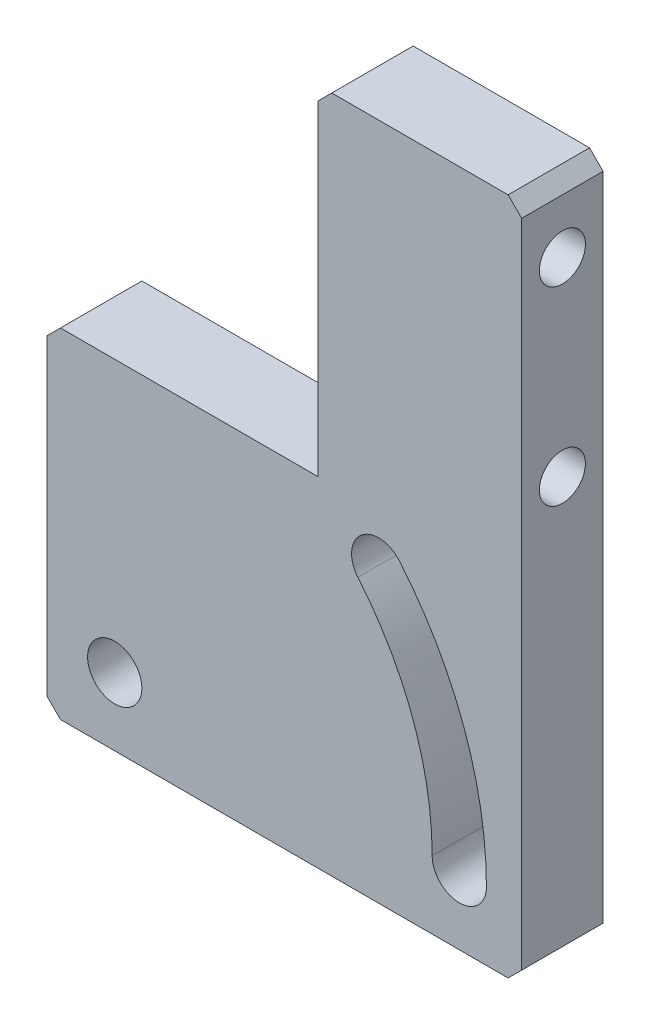
SolidWorks part; units mm, degrees
material "AL6061"
ref_plane "前视基准面" through (0, 0, 0) normal (0, 0, 1) x (1, 0, 0)
ref_plane "上视基准面" through (0, 0, 0) normal (0, 1, 0) x (1, 0, 0)
ref_plane "右视基准面" through (0, 0, 0) normal (1, 0, 0) x (0, 0, -1)
sketch "草图1" plane through (0, 0, 0) normal (0, 0, 1) x (1, 0, 0)
  line L1 (17.5, -25) -> (-17.5, -25)
  line L2 (17.5, -25) -> (17.5, 25)
  line L3 (17.5, 25) -> (-17.5, 25)
  line L4 (-17.5, -25) -> (-17.5, 25)
  line L5 (17.5, -25) -> (-17.5, 25) construction
  line L6 (17.5, 25) -> (-17.5, -25) construction
  point P0 (0, 0)
  dimension "D1" = 35
  dimension "D2" = 50
extrude "凸台-拉伸1" add sketch "草图1" along normal mid plane 6
sketch "草图2" plane through (0, 0, 3) normal (0, 0, 1) x (1, 0, 0)
  line L0 (17.5, -25) -> (17.5, 25) construction
  line L1 (-17.5, 25) -> (2.5, 25)
  line L2 (-17.5, 25) -> (-17.5, 0)
  line L3 (-17.5, 0) -> (2.5, 0)
  line L4 (2.5, 25) -> (2.5, 0)
  dimension "D1" = 15
  dimension "D2" = 25
extrude "切除-拉伸1" cut sketch "草图2" against normal through all
sketch "草图3" plane through (0, 0, 3) normal (0, 0, 1) x (1, 0, 0)
  line L0 (-17.5, 0) -> (-17.5, -25) construction
  line L1 (-17.5, -25) -> (17.5, -25) construction
  line L2 (-12.5, -20) -> (11.3682, -11.3127) construction
  line L3 (-12.5, -20) -> (0.9382, -20) construction
  line L4 (-12.5, -20) -> (12.9, -20) construction
  line L5 (-12.5, -20) -> (6.9575, -3.6732) construction
  circle A0 centre (-12.5, -20) radius 2
  arc A1 (6.9575, -3.6732) -> (12.9, -20) centre (-12.5, -20) cw construction
  arc A2 (14.9, -20) -> (8.4896, -2.3876) centre (-12.5, -20) ccw
  arc A3 (10.9, -20) -> (5.4254, -4.9588) centre (-12.5, -20) ccw
  arc A4 (10.9, -20) -> (14.9, -20) centre (12.9, -20) ccw
  arc A5 (8.4896, -2.3876) -> (5.4254, -4.9588) centre (6.9575, -3.6732) ccw
  point P4 (11.3682, -11.3127)
  dimension "D1" = 4
  dimension "D2" = 5
  dimension "D3" = 5
  dimension "D4" = 25.4
  dimension "D5" = 20
  dimension "D6" = 40
extrude "切除-拉伸2" cut sketch "草图3" against normal through all
sketch "草图4" plane through (2.5, 0, 0) normal (-1, 0, 0) x (0, 0, 1)
  line L0 (0, 25) -> (0, 20) construction
  line L1 (-3, 25) -> (3, 25) construction
  line L2 (0, 20) -> (0, 6) construction
  point P0 (0, 20)
  point P2 (0, 6)
  dimension "D1" = 5
  dimension "D2" = 14
hole_wizard "M3 间隙孔1" positions "草图4" profile "草图6" hole size "M3" standard "ISO" end condition through all
sketch "草图6" plane through (2.5, 20, 0) normal (0, 1, 0) x (0, 0, 1)
  line L0 (0, 0) -> (0, 15)
  line L1 (0, 15) -> (1.7, 15)
  line L2 (1.7, 15) -> (1.7, 0)
  line L5 (1.7, 0) -> (0, 0)
  line L11 (0, -6.35) -> (0, 107.95) construction
  dimension "通孔孔直径" = 3.4
  dimension "通孔孔深度" = 15
chamfer "倒角1" distance 1 angle 45 5 edges at (17.5, -25, 0) (17.5, 25, 0) (2.5, 25, 0) (-17.5, -25, 0) (-17.5, 0, 0)
